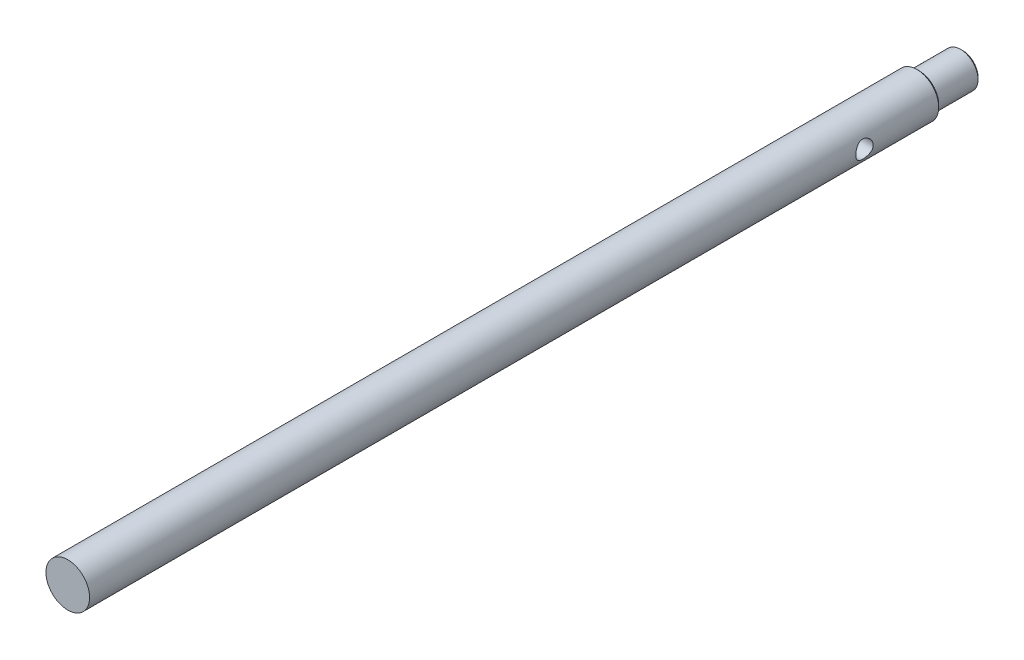
from build123d import *

# Parameters (mm, degrees)
SKETCH2_W               = 150
SKETCH2_H               = 10
CUT_EXTRUDE1_DEPTH      = 10
CUT_EXTRUDE1_DEPTH_BACK = 10
SKETCH5_R               = 4
SKETCH6_R               = 10
BOSS_EXTRUDE1_DEPTH     = 20
SKETCH7_R               = 8
BOSS_EXTRUDE2_DEPTH     = 20
CHAMFER1_SIZE           = 1
BOSS_EXTRUDE4_START     = 220
SKETCH8_R               = 10
BOSS_EXTRUDE4_DEPTH     = 220


with BuildPart() as part:
    # Sketch2 → Revolve4 (revolve)
    with BuildSketch(Plane(origin=(0, 0, 0), x_dir=(0, 0, -1), z_dir=(1, 0, 0)), mode=Mode.PRIVATE) as revolve4_sk:
        with Locations((75, 5)):
            Rectangle(SKETCH2_W, SKETCH2_H)
    revolve(revolve4_sk.sketch.rotate(Axis((0, 0, 0), (0, 0, -1)), 90), axis=Axis((0, 0, 0), (0, 0, -1)))

    # Sketch5 → Cut-Extrude1 (cut, two sides: drawn at the far end of the back side and taken through both)
    with BuildSketch(Plane(origin=(0, 0, 0), x_dir=(0, 0, -1), z_dir=(1, 0, 0)).offset(-CUT_EXTRUDE1_DEPTH_BACK)):
        with Locations(Location((135, 0, 0), (0, 0, 180))):
            Circle(SKETCH5_R)
    extrude(amount=CUT_EXTRUDE1_DEPTH + CUT_EXTRUDE1_DEPTH_BACK, mode=Mode.SUBTRACT)

    # Sketch6 → Boss-Extrude1 (add)
    with BuildSketch(Plane(origin=(0, 0, -150), x_dir=(-1, 0, 0), z_dir=(0, 0, -1))):
        with Locations(Location((0, 0, 0), (0, 0, 180))):
            Circle(SKETCH6_R)
    extrude(amount=BOSS_EXTRUDE1_DEPTH)

    # Sketch7 → Boss-Extrude2 (add)
    with BuildSketch(Plane(origin=(0, 0, -170), x_dir=(-1, 0, 0), z_dir=(0, 0, -1))):
        Circle(SKETCH7_R)
    extrude(amount=BOSS_EXTRUDE2_DEPTH)

    # Chamfer1
    chamfer1_edges = [part.edges().sort_by_distance(p)[0] for p in [
        (-10, 0, -170),
        (8, 0, -190),
    ]]
    chamfer(chamfer1_edges, length=CHAMFER1_SIZE)

    # Sketch8 → Boss-Extrude4 (add)
    with BuildSketch(Plane.XY.offset(BOSS_EXTRUDE4_START)):
        Circle(SKETCH8_R)
    extrude(amount=-BOSS_EXTRUDE4_DEPTH)


solid = part.part
